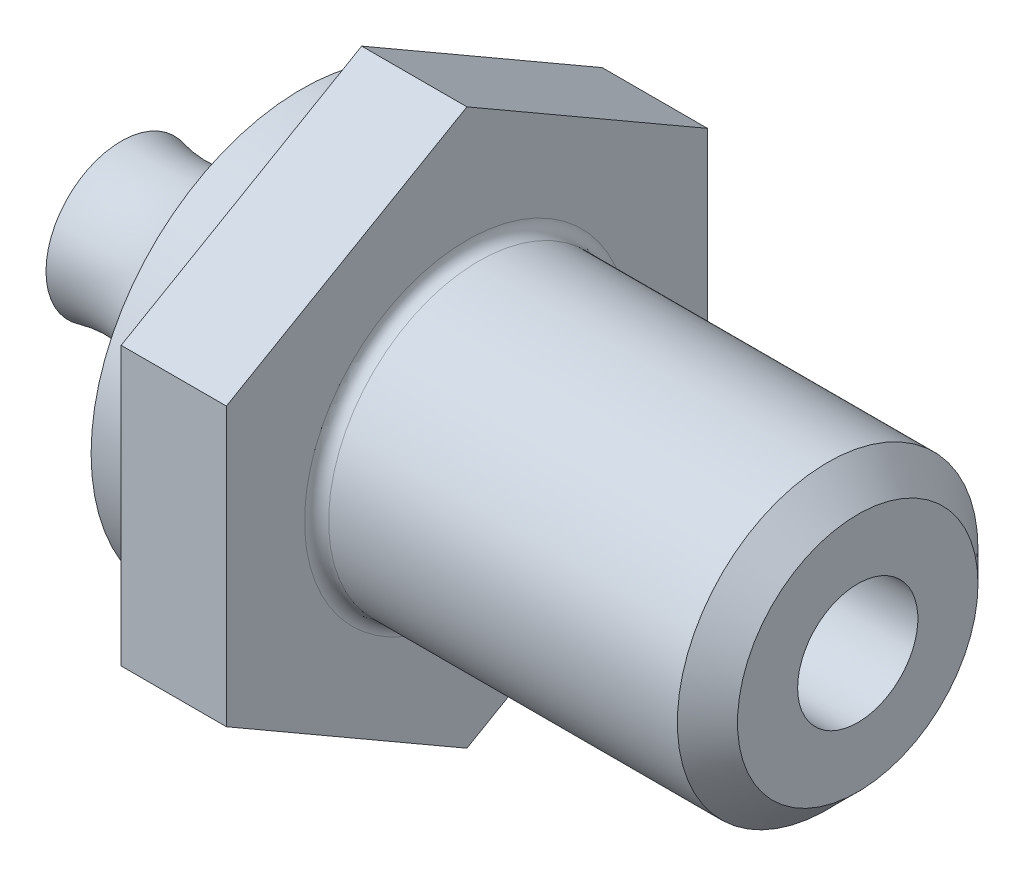
SolidWorks part; units mm, degrees
ref_plane "Front Plane" through (0, 0, 0) normal (0, 0, 1) x (1, 0, 0)
ref_plane "Top Plane" through (0, 0, 0) normal (0, 1, 0) x (1, 0, 0)
ref_plane "Right Plane" through (0, 0, 0) normal (1, 0, 0) x (0, 0, -1)
sketch "Sketch1" plane through (0, 0, 0) normal (1, 0, 0) x (0, 0, -1)
  line L0 (8, 4.6188) -> (8, -4.6188)
  line L1 (-8, 4.6188) -> (-8, -4.6188)
  line L2 (8, -4.6188) -> (0, -9.2376)
  line L3 (0, -9.2376) -> (-8, -4.6188)
  line L4 (8, 4.6188) -> (0, 9.2376)
  line L5 (0, 9.2376) -> (-8, 4.6188)
  dimension "s" = 16
  dimension "D2" = 120
  dimension "D3" = 8
  dimension "D4" = 8
  dimension "D5" = 8
extrude "Base-Extrude" add sketch "Sketch1" along normal blind 6.4
sketch "Sketch2" plane through (0, 0, 0) normal (0, 0, 1) x (1, 0, 0)
  line L0 (0, 4.6188) -> (0, -4.6188) construction
  line L1 (0, 0) -> (32.4, 0)
  line L2 (0, 0) -> (0, 5)
  line L3 (0, 5) -> (27.8072, 5)
  line L4 (32.4, 0) -> (32.4, 4.134)
  line L5 (6.4, 9.2376) -> (6.4, 4.6188) construction
  line L7 (0, 0) -> (96.52, 0) construction
  line L8 (32.4, -4.134) -> (27.8072, -5) construction
  line L9 (0, -5) -> (27.8072, -5) construction
  line L10 (7.4, 15.24) -> (7.4, -1.27) construction
  line L11 (6.4, 15.24) -> (6.4, -1.27) construction
  line L12 (6.4, 4.6188) -> (6.4, -4.6188) construction
  line L13 (27.8072, 5) -> (32.4, 5)
  line L14 (32.4, 5) -> (32.4, 4.134)
  dimension "l" = 26
  dimension "m" = 10
  dimension "Minor_dia" = 8.268
  dimension "p" = 1
  dimension "h" = 26
revolve "Boss-Revolve1" add sketch "Sketch2" angle 360 about L7
cosmetic thread "Helix line 1" parameters "Thread_length"=25, "Thread_minor"=8.268
sketch "Sketch3" plane through (0, 0, 0) normal (0, 0, 1) x (1, 0, 0)
  line L0 (0, 8) -> (3.6013, 14.2376)
  line L1 (0, 9.2376) -> (0, 4.6188) construction
  line L2 (3.6013, 14.2376) -> (3.6013, 19.2376)
  line L3 (3.6013, 19.2376) -> (-10, 19.2376)
  line L4 (-10, 19.2376) -> (-10, 8)
  line L5 (-10, 8) -> (0, 8)
  line L6 (0, 0) -> (99.06, 0) construction
  line L7 (6.4, 9.2376) -> (0, 9.2376) construction
  dimension "D1" = 8
  dimension "D2" = 5
  dimension "D3" = 10
  dimension "D4" = 5
  dimension "Head_ch_ang" = 30
revolve "Cut-Revolve1" cut sketch "Sketch3" angle 360 about L6
sketch "Sketch5" plane through (0, 0, 0) normal (0, 0, 1) x (1, 0, 0)
  line L0 (6.4, 8) -> (2.7987, 14.2376)
  line L1 (6.4, 9.2376) -> (6.4, 4.6188) construction
  line L2 (2.7987, 14.2376) -> (2.7987, 19.2376)
  line L3 (2.7987, 19.2376) -> (12.7987, 19.2376)
  line L4 (12.7987, 19.2376) -> (12.7987, 8)
  line L5 (12.7987, 8) -> (6.4, 8)
  line L7 (6.4, 9.2376) -> (0.7145, 9.2376) construction
  line L8 (0, 0) -> (99.06, 0) construction
  line L9 (0, 0) -> (99.06, 0) construction
  dimension "D1" = 8
  dimension "D2" = 5
  dimension "D3" = 10
  dimension "Head_ch_ang" = 30
  dimension "D4" = 5
revolve "Cut-Revolve2" [suppressed] cut sketch "Sketch5" angle 360 about L8
sketch "Sketch4" plane through (0, 0, 0) normal (0, 0, 1) x (1, 0, 0)
  line L1 (6.4, 9.2376) -> (6.4, 4.6188) construction
  line L2 (6.4, 8) -> (5.8, 8)
  line L3 (6.4, 8) -> (6.4, 19.2376)
  line L4 (6.4, 19.2376) -> (5.8, 19.2376)
  line L5 (0, 0) -> (95.25, 0) construction
  line L6 (0, 0) -> (96.52, 0) construction
  line L7 (5.8, 8) -> (5.8, 19.2376)
  line L8 (6.4, 9.2376) -> (0.7145, 9.2376) construction
  dimension "D1" = 16
  dimension "D2" = 10
  dimension "c" = 0.6
revolve "Cut-Revolve3" [suppressed] cut sketch "Sketch4" angle 360 about L5
chamfer "Chamfer" [suppressed] distance 0.8 angle 45
fillet "Fillet" radius 0.4 1 edges at (6.4, 0, -5)
sketch "Sketch6" plane through (0, 0, 0) normal (0, 0, 1) x (1, 0, 0)
  line L0 (7.4, -4.134) -> (6.9, -5)
  line L1 (7.4, -4.134) -> (7.9, -5)
  line L2 (7.9, -5) -> (7.9, -6.25)
  line L3 (-3.175, 0) -> (5.1513, 0) construction
  line L5 (7.9, -6.25) -> (6.9, -6.25)
  line L6 (6.9, -6.25) -> (6.9, -5)
  dimension "Thread_minor" = 8.268
  dimension "Diameter" = 10
  dimension "Start" = 7.4
  dimension "SideAngle" = 60
  dimension "VeeAngle" = 60
  dimension "Overcut" = 12.5
revolve "Cut-Revolve4" [suppressed] cut sketch "Sketch6" angle 360 about L3
pattern_linear "LPattern1" [suppressed]
sketch "Sketch7" plane through (0, 0, 0) normal (0, 1, 0) x (1, 0, 0)
  line L0 (32.4, 5) -> (18.4, 5)
  line L1 (32.4, -5) -> (32.4, 5) construction
  line L2 (32.4, 5) -> (6.8, 5) construction
  line L3 (18.4, 5) -> (19.4, 4)
  line L4 (19.4, 4) -> (19.4, 0)
  line L5 (19.4, 0) -> (32.4, 0)
  line L6 (32.4, 0) -> (32.4, 5)
  line L7 (34.2095, 0) -> (7.5705, 0) construction
  dimension "D1" = 45
  dimension "D2" = 13
  dimension "D3" = 1
revolve "Cut-Revolve5" cut sketch "Sketch7" angle 360 about L7
sketch "Sketch8" plane through (0, 0, 0) normal (0, 1, 0) x (1, 0, 0)
  line L0 (6.4, -8) -> (0.7145, -8) construction
  line L1 (0, 8) -> (2.9, 8)
  line L2 (0, 8) -> (0, -8)
  line L3 (0, -8) -> (2.9, -8)
  line L4 (2.9, 8) -> (2.9, -8)
  line L5 (6.4, 8) -> (6.4, 0) construction
  line L6 (0, 8) -> (0, 4) construction
  line L7 (6.4, 8) -> (0.7145, 8) construction
  dimension "D1" = 3.5
extrude "Cut-Extrude1" cut sketch "Sketch8" against normal through all and the other way through all
sketch "Sketch9" plane through (0, 0, 0) normal (0, 1, 0) x (1, 0, 0)
  line L0 (-7.3175, 0) -> (20.7389, 0) construction
  line L1 (-5.1, 0) -> (-5.1, 2.5)
  line L2 (0.9, 6) -> (0.9, 7)
  line L3 (2.9, 0) -> (2.9, -8) construction
  line L4 (0.9, 7) -> (2.9, 7)
  line L5 (2.9, 8) -> (2.9, 0) construction
  line L7 (2.9, 7) -> (2.9, 0)
  line L8 (2.9, 0) -> (-5.1, 0)
  arc A0 (-5.1, 2.5) -> (0.9, 6) centre (-3.9124, 7.3569) ccw
  point P6 (-5.1, 0)
  point P18 (2.9, 0)
  dimension "D3" = 5
  dimension "D1" = 5
  dimension "D2" = 2
  dimension "D4" = 8
  dimension "D5" = 14
  dimension "D6" = 1
revolve "Revolve1" add sketch "Sketch9" angle 360 about L0
sketch "Sketch10" plane through (0, 0, 0) normal (0, 1, 0) x (1, 0, 0)
  line L0 (-5.7992, 0) -> (20.0578, 0) construction
  line L1 (19.4, 0) -> (19.4, 2)
  line L2 (19.4, -4) -> (19.4, 4) construction
  line L3 (19.4, 2) -> (-0.2247, 2)
  line L4 (-0.2247, 2) -> (-0.2247, 1.5)
  line L5 (-0.2247, 1.5) -> (-4.1, 1.5)
  line L6 (-5.1, 2.5) -> (-5.1, -2.5) construction
  line L7 (-5.1, 1.118) -> (-5.1, 0)
  line L8 (-5.1, 0) -> (19.4, 0)
  arc A0 (-5.1, 1.118) -> (-4.1, 1.5) centre (-4.1, 0) cw
  dimension "D1" = 1.5
  dimension "D2" = 1
  dimension "D3" = 4
revolve "Cut-Revolve6" cut sketch "Sketch10" angle 360 about L0
